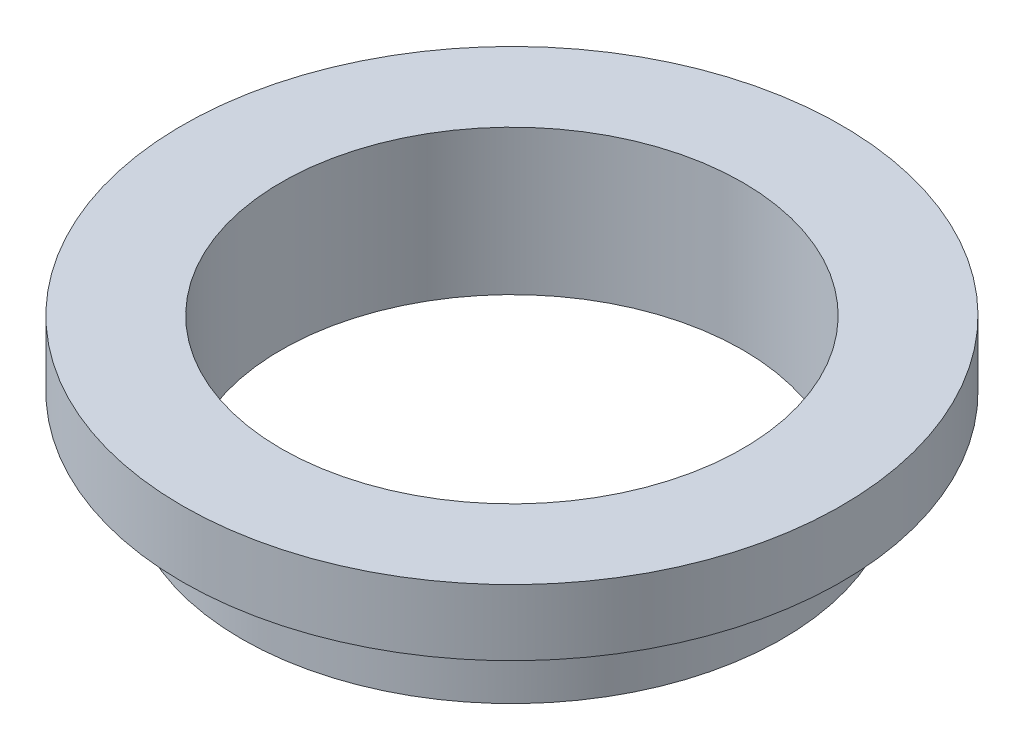
from build123d import *


with BuildPart() as part:
    # 草图1 → 旋转1 (revolve)
    with BuildSketch(Plane(origin=(0, 0, 0), x_dir=(0, 0, -1), z_dir=(1, 0, 0)), mode=Mode.PRIVATE) as revolve_1_sk:
        Polygon((17.5, 0), (17.5, 11), (25, 11), (25, 6), (20.5, 6), (20.5, 0), align=None)
    revolve(revolve_1_sk.sketch.rotate(Axis((0, 46.271659978, 0), (0, -1, 0)), 180), axis=Axis((0, 46.271659978, 0), (0, -1, 0)))


solid = part.part
